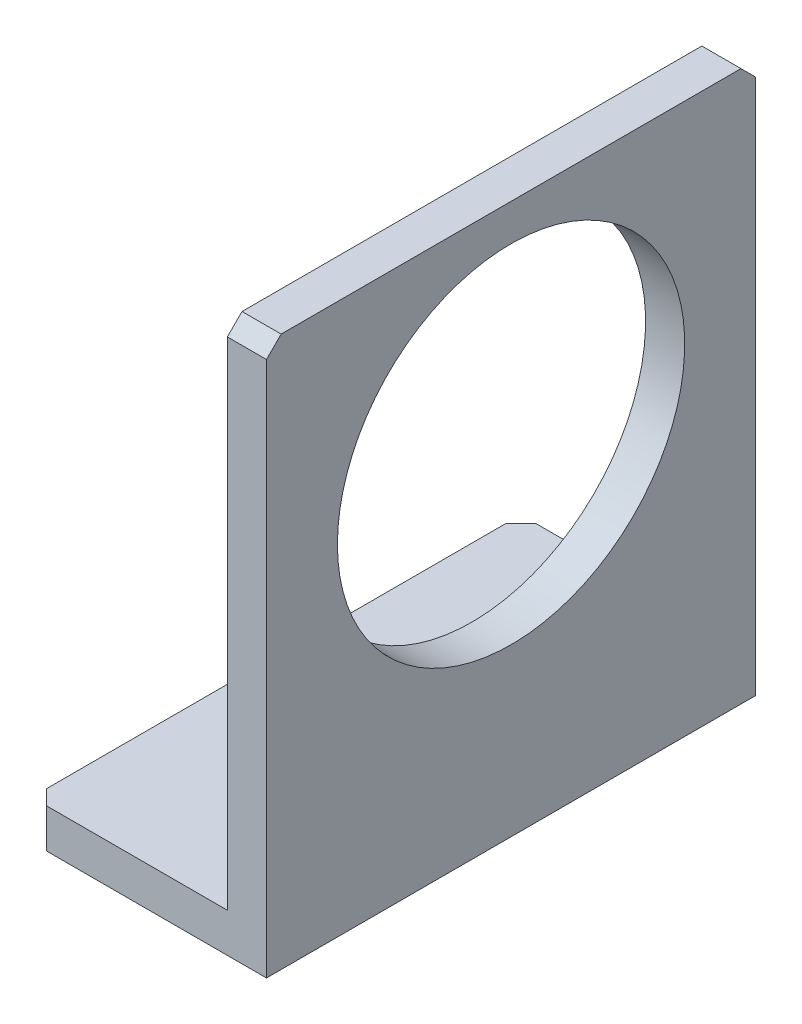
from build123d import *

# Parameters (mm, degrees)
EXTRUDE_1_DEPTH     = 50
CHAMFER_1_SIZE      = 3
CUT_EXTRUDE_1_REACH = 148.206
SKETCH_4_R          = 35.5


with BuildPart() as part:
    # 草图2 → 凸台-拉伸1 (new, symmetric)
    with BuildSketch(Plane(origin=(409.637600706, 0.5, -34.379468655), x_dir=(1, 0, 0), z_dir=(0, 0, 1))):
        Polygon((-409.637600706, 112), (-409.637600706, -0.5), (-457.637600706, -0.5), (-457.637600706, 7.5), (-417.637600706, 7.5), (-417.637600706, 112), align=None)
    extrude(amount=EXTRUDE_1_DEPTH, both=True)

    # 倒角1
    chamfer_1_edges = [part.edges().sort_by_distance(p)[0] for p in [
        (-48, 4, 15.620531345),
        (-4, 112.5, 15.620531345),
        (-48, 4, -84.379468655),
        (-4, 112.5, -84.379468655),
    ]]
    chamfer(chamfer_1_edges, length=CHAMFER_1_SIZE)

    # 草图4 → 切除-拉伸1 (cut, up to next)
    with BuildSketch(Plane.ZY.offset(8), mode=Mode.PRIVATE) as cut_extrude_1_sk1:
        with Locations((-34.379468655, 69.5)):
            Circle(SKETCH_4_R)
    cut_extrude_1_tool1 = extrude(cut_extrude_1_sk1.sketch, amount=-CUT_EXTRUDE_1_REACH, mode=Mode.PRIVATE) & part.part
    add(cut_extrude_1_tool1.solids().sort_by_distance((-8, 69.5, -34.379469))[0], mode=Mode.SUBTRACT)


solid = part.part
